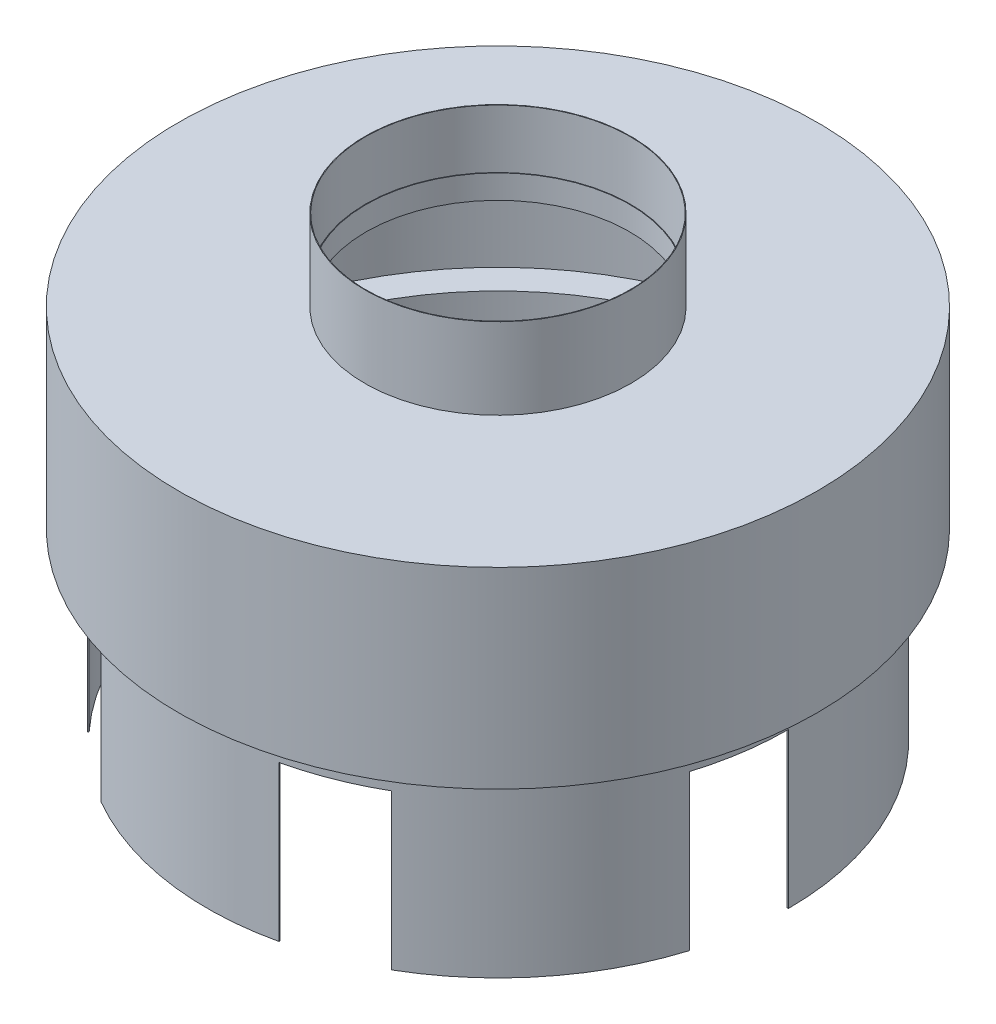
from build123d import *

# Parameters (mm, degrees)
SHELL1_T           = -2
SKETCH2_R          = 229
CUT_EXTRUDE1_DEPTH = 101
CUT_EXTRUDE2_DEPTH = 268
CIRPATTERN1_COUNT  = 6


with BuildPart() as part:
    # Sketch1 → Revolve1 (revolve)
    with BuildSketch(Plane.XY):
        Polygon((0, 0), (0, 790), (230, 790), (230, 650), (552, 650), (552, 318), (502, 318), (502, 0), align=None)
    revolve(axis=Axis((0, 0, 0), (0, 1, 0)))

    # Shell1
    shell1_openings = [part.faces().sort_by_distance(p)[0] for p in [
        (0, 0, 0),
    ]]
    offset(amount=SHELL1_T, openings=shell1_openings, kind=Kind.INTERSECTION)

    # Sketch2 → Cut-Extrude1 (cut)
    with BuildSketch(Plane(origin=(0, 790, 0), x_dir=(1, 0, 0), z_dir=(0, 1, 0))):
        with Locations(Location((0, 0, 0), (0, 0, 180))):
            Circle(SKETCH2_R)
    extrude(amount=-CUT_EXTRUDE1_DEPTH, mode=Mode.SUBTRACT)

    # Sketch3 → Cut-Extrude2 (cut)
    with BuildSketch(Plane(origin=(0, 0, 0), x_dir=(1, 0, 0), z_dir=(0, 1, 0))):
        Polygon((0, 0), (635.384163394, 0), (612.361562027, -189.37712274), align=None)
    cut_extrude2 = extrude(amount=CUT_EXTRUDE2_DEPTH, mode=Mode.SUBTRACT)

    # CirPattern1: Cut-Extrude2 ×6 about axis
    cirpattern1_axis = Axis((0, 0, 0), (0, 1, 0))
    for i in range(1, CIRPATTERN1_COUNT):
        add(cut_extrude2.rotate(cirpattern1_axis, i * 360 / CIRPATTERN1_COUNT), mode=Mode.SUBTRACT)


solid = part.part
